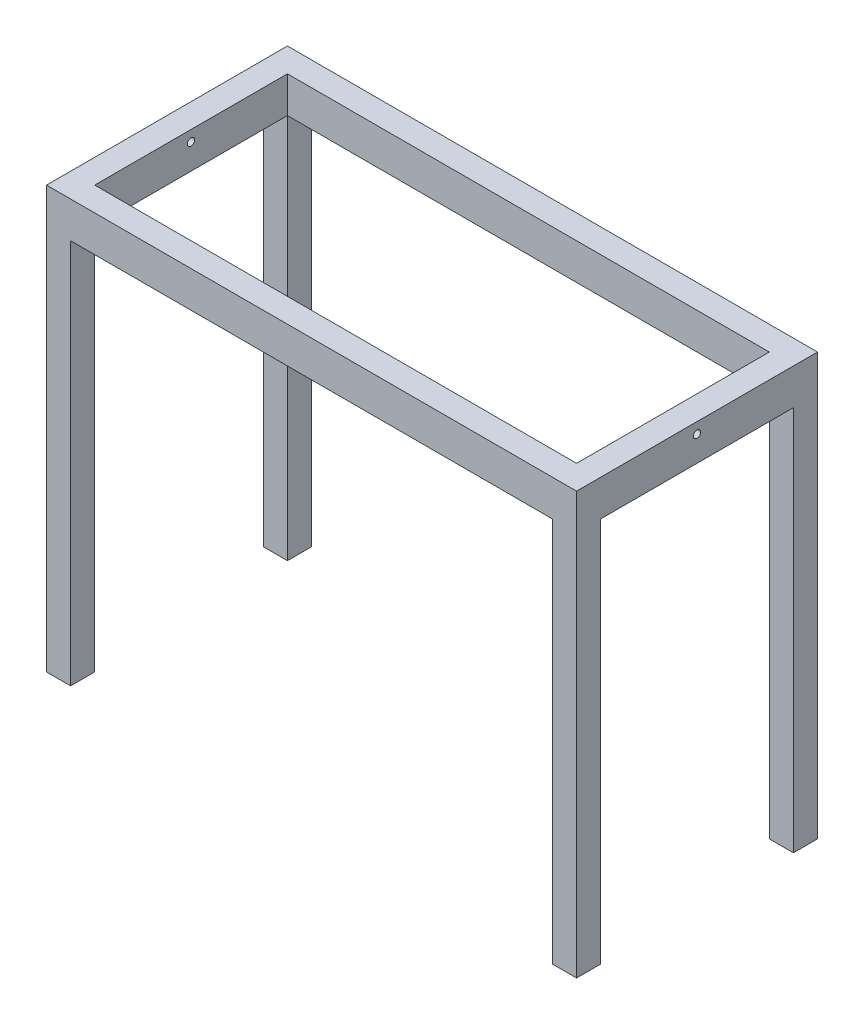
SolidWorks part; units mm, degrees
ref_plane "Front Plane" through (0, 0, 0) normal (0, 0, 1) x (1, 0, 0)
ref_plane "Top Plane" through (0, 0, 0) normal (0, 1, 0) x (1, 0, 0)
ref_plane "Right Plane" through (0, 0, 0) normal (1, 0, 0) x (0, 0, -1)
other "Configuration Table"
sketch "Sketch1" plane through (0, 0, 0) normal (0, 1, 0) x (1, 0, 0)
  line L1 (-500, -200) -> (500, -200)
  line L2 (-500, -200) -> (-500, 200)
  line L3 (-500, 200) -> (500, 200)
  line L4 (500, -200) -> (500, 200)
  line L5 (-500, -200) -> (500, 200) construction
  line L6 (-500, 200) -> (500, -200) construction
  line L7 (-550, -250) -> (550, -250)
  line L8 (-550, -250) -> (-550, 250)
  line L9 (-550, 250) -> (550, 250)
  line L10 (550, -250) -> (550, 250)
  line L11 (-550, -250) -> (550, 250) construction
  line L12 (-550, 250) -> (550, -250) construction
  point P0 (0, 0)
  point P6 (0, 0)
  dimension "D1" = 1100
  dimension "D2" = 500
  dimension "D3" = 1000
  dimension "D4" = 400
extrude "Boss-Extrude1" add sketch "Sketch1" along normal blind 75
sketch "Sketch2" plane through (0, 0, 0) normal (0, -1, 0) x (1, 0, 0)
  line L0 (-500, -200) -> (-500, 200) construction
  line L1 (-550, 250) -> (-500, 250)
  line L2 (-550, 250) -> (-550, 200)
  line L3 (-550, 200) -> (-500, 200)
  line L4 (-500, 250) -> (-500, 200)
  line L5 (0, 0) -> (0, 293.5078) construction
  line L6 (-500, 200) -> (500, 200) construction
  line L7 (500, 250) -> (500, 200)
  line L8 (550, 200) -> (500, 200)
  line L9 (550, 250) -> (550, 200)
  line L10 (550, 250) -> (500, 250)
  line L11 (0, 0) -> (140.0572, 0) construction
  line L12 (550, -250) -> (500, -250)
  line L13 (550, -250) -> (550, -200)
  line L14 (550, -200) -> (500, -200)
  line L15 (500, -250) -> (500, -200)
  line L16 (-500, -250) -> (-500, -200)
  line L17 (-550, -200) -> (-500, -200)
  line L18 (-550, -250) -> (-550, -200)
  line L19 (-550, -250) -> (-500, -250)
extrude "Boss-Extrude2" add sketch "Sketch2" along normal blind 800
sketch "Sketch3" plane through (-550, 0, 0) normal (-1, 0, 0) x (0, 0, 1)
  line L0 (0, 75) -> (0, 0) construction
  line L1 (-250, 75) -> (250, 75) construction
  line L2 (-200, 0) -> (200, 0) construction
  circle A0 centre (0, 52.5) radius 7.5
  dimension "D1" = 15
  dimension "D2" = 22.5
extrude "Cut-Extrude1" cut sketch "Sketch3" against normal through all both and the other way through all
